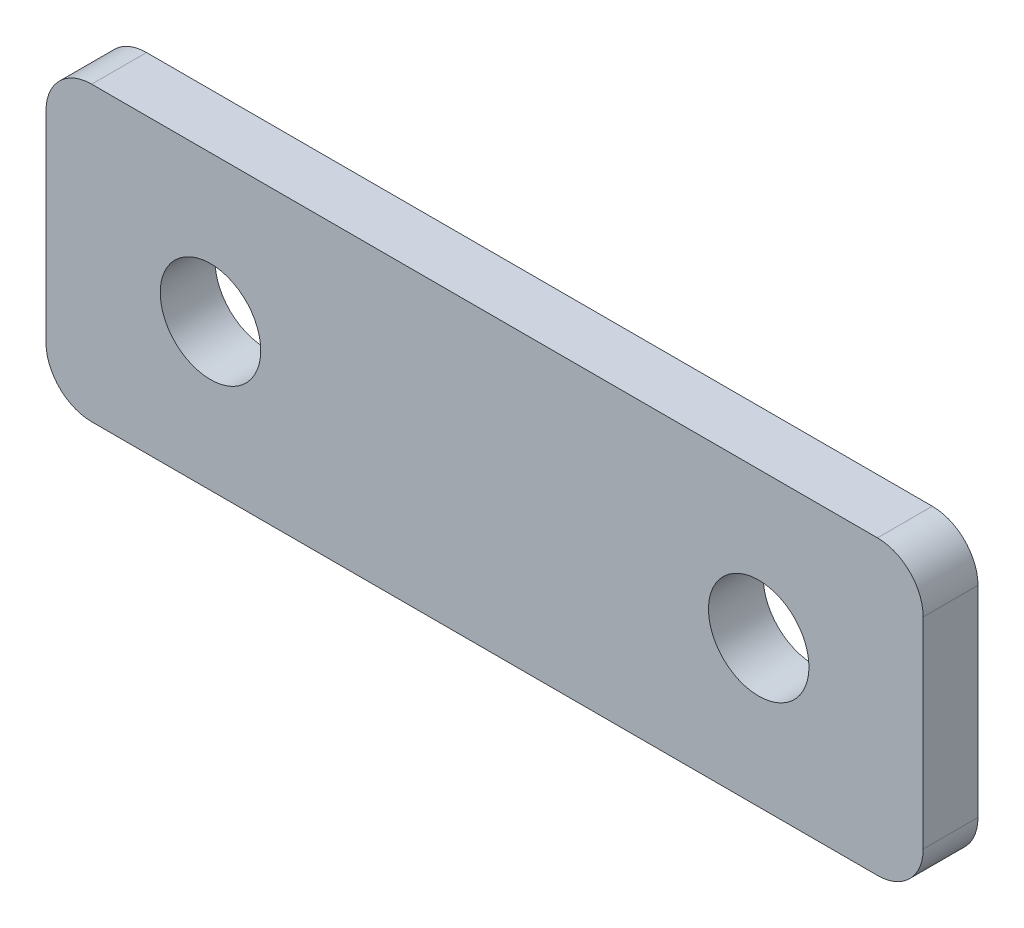
from build123d import *

# Parameters (mm, degrees)
SKETCH1_W           = 96
SKETCH1_H           = 32
BOSS_EXTRUDE1_DEPTH = 6
FILLET1_R           = 5
SKETCH2_R           = 5.5
CUT_EXTRUDE1_DEPTH  = 6
LPATTERN1_COUNT     = 2
LPATTERN1_PITCH     = 60


with BuildPart() as part:
    # Sketch1 → Boss-Extrude1 (new body)
    with BuildSketch(Plane.XY):
        with Locations((48, -16)):
            Rectangle(SKETCH1_W, SKETCH1_H)
    extrude(amount=BOSS_EXTRUDE1_DEPTH)

    # Fillet1
    fillet1_edges = [part.edges().sort_by_distance(p)[0] for p in [
        (0, 0, 3),
        (96, 0, 3),
        (96, -32, 3),
        (0, -32, 3),
    ]]
    fillet(fillet1_edges, radius=FILLET1_R)

    # Sketch2 → Cut-Extrude1 (cut)
    with BuildSketch(Plane.XY.offset(6)):
        with Locations((18, -16)):
            Circle(SKETCH2_R)
    cut_extrude1 = extrude(amount=-CUT_EXTRUDE1_DEPTH, mode=Mode.SUBTRACT)

    # LPattern1: Cut-Extrude1 ×2
    with Locations(*[(i * LPATTERN1_PITCH, 0, 0) for i in range(1, LPATTERN1_COUNT)]):
        add(cut_extrude1, mode=Mode.SUBTRACT)


solid = part.part
